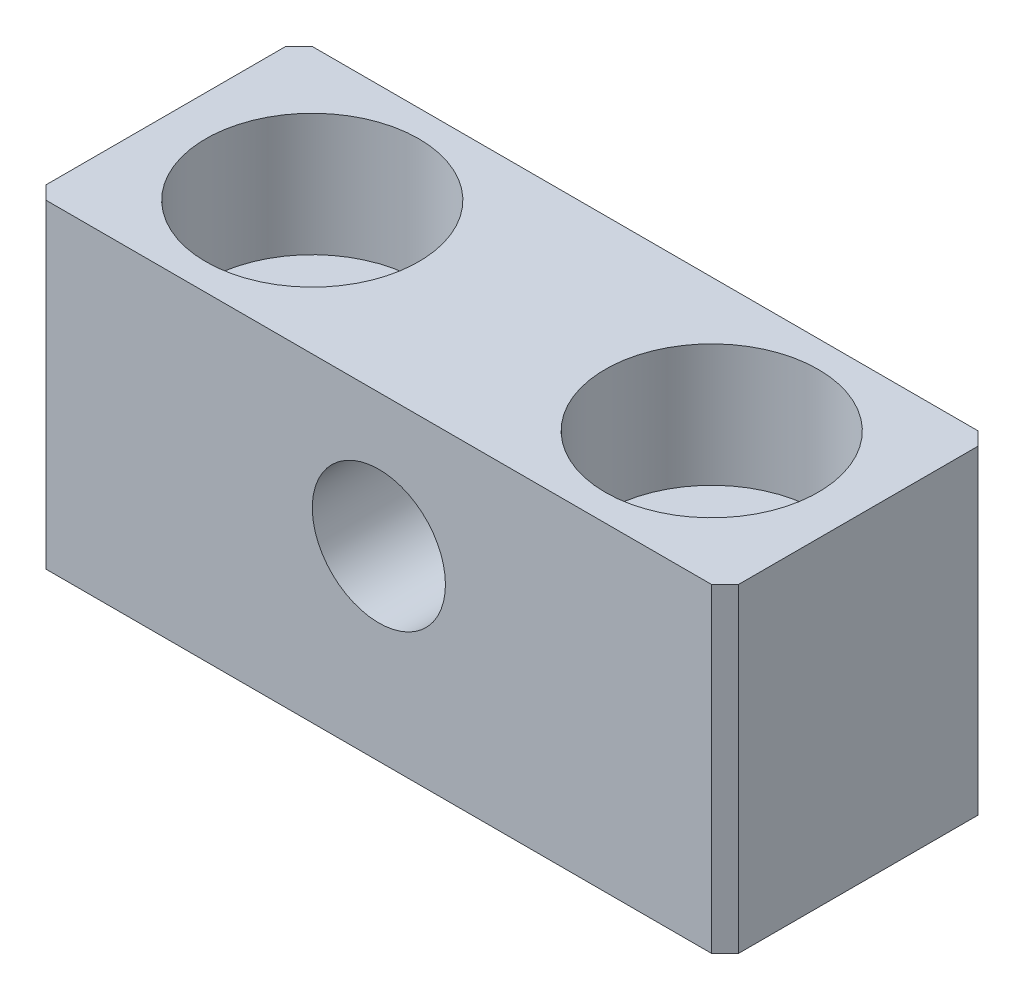
from build123d import *

# Parameters (mm, degrees)
SKETCH_1_W                = 26
SKETCH_1_H                = 12
EXTRUDE_1_DEPTH           = 5
HOLE_WIZARD_1_D           = 4.5
HOLE_WIZARD_1_CBORE_D     = 8
HOLE_WIZARD_1_CBORE_DEPTH = 4.6
HOLE_WIZARD_M6_1_D        = 5
CHAMFER_1_SIZE            = 0.5


with BuildPart() as part:
    # 草图1 → 凸台-拉伸1 (new, symmetric)
    with BuildSketch(Plane.XY):
        Rectangle(SKETCH_1_W, SKETCH_1_H)
    extrude(amount=EXTRUDE_1_DEPTH, both=True)

    # 打孔尺寸(%根据)内六角圆柱头螺钉的类型1 (through all)
    with Locations(Plane(origin=(0, 6, 0), x_dir=(1, 0, 0), z_dir=(0, 1, 0))):
        with Locations((-7.5, 0), (7.5, 0)):
            CounterBoreHole(HOLE_WIZARD_1_D / 2, HOLE_WIZARD_1_CBORE_D / 2, HOLE_WIZARD_1_CBORE_DEPTH)

    # M6 螺纹孔1 (through all)
    with Locations(Plane.XY.offset(5)):
        with Locations((0, 1)):
            Hole(HOLE_WIZARD_M6_1_D / 2)

    # 倒角1
    chamfer_1_edges = [part.edges().sort_by_distance(p)[0] for p in [
        (-13, 0, 5),
        (13, 0, 5),
        (-13, 0, -5),
        (13, 0, -5),
    ]]
    chamfer(chamfer_1_edges, length=CHAMFER_1_SIZE)


solid = part.part
